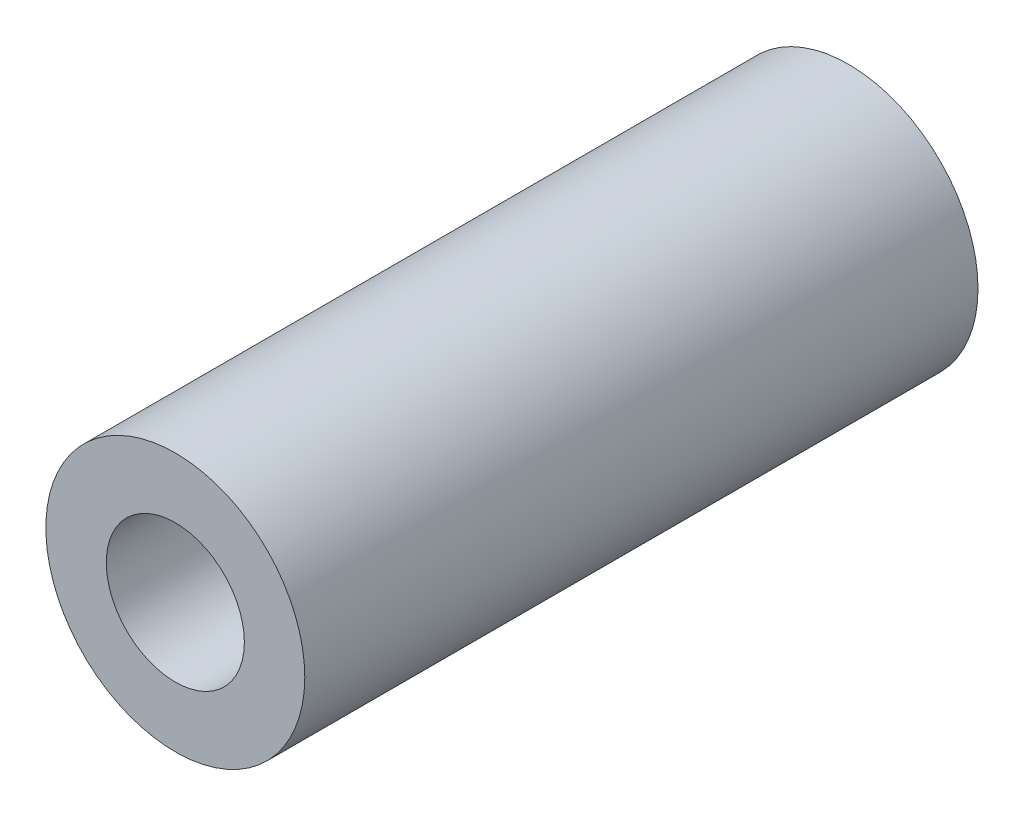
SolidWorks part; units mm, degrees
ref_plane "Front Plane" through (0, 0, 0) normal (0, 0, 1) x (1, 0, 0)
ref_plane "Top Plane" through (0, 0, 0) normal (0, 1, 0) x (1, 0, 0)
ref_plane "Right Plane" through (0, 0, 0) normal (1, 0, 0) x (0, 0, -1)
sketch "Sketch1" plane through (0, 0, 0) normal (0, 0, 1) x (1, 0, 0)
  circle A0 centre (0, 0) radius 4
  circle A1 centre (0, 0) radius 7.5
  dimension "D1" = 8
  dimension "D2" = 15
extrude "Boss-Extrude1" add sketch "Sketch1" along normal blind 39
